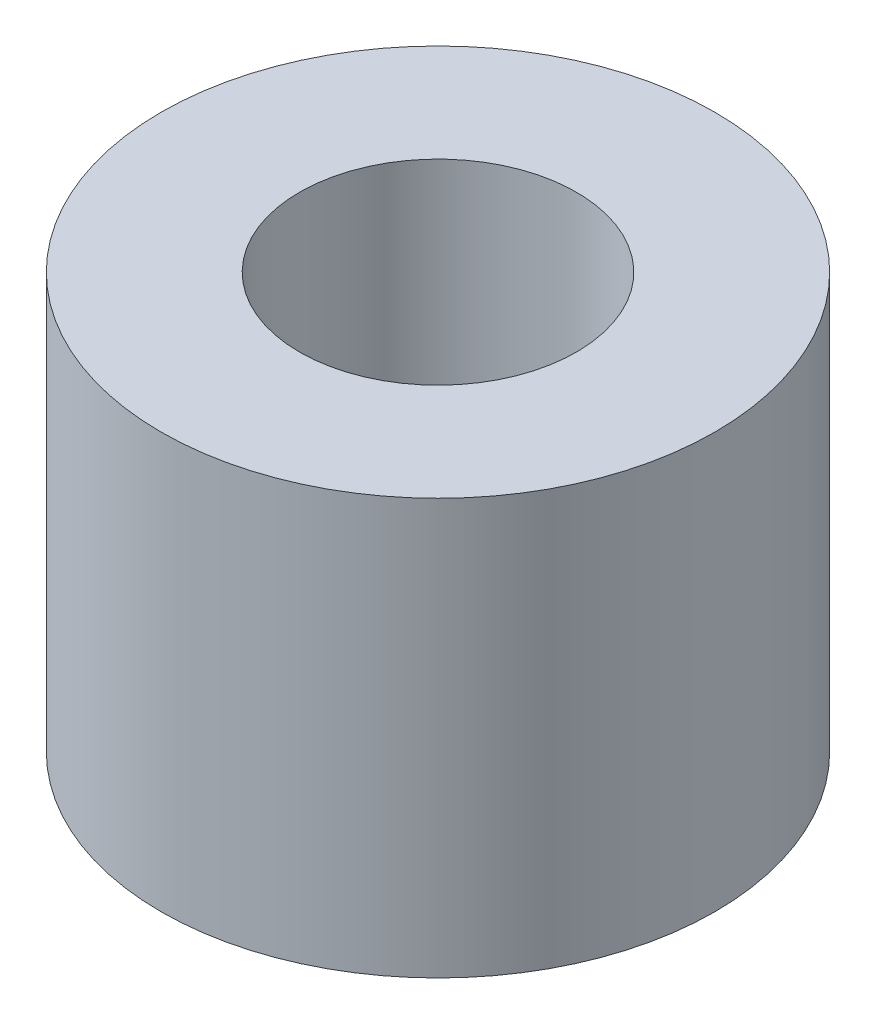
SolidWorks part; units mm, degrees
material "ABS"
ref_plane "Front Plane" through (0, 0, 0) normal (0, 0, 1) x (1, 0, 0)
ref_plane "Top Plane" through (0, 0, 0) normal (0, 1, 0) x (1, 0, 0)
ref_plane "Right Plane" through (0, 0, 0) normal (1, 0, 0) x (0, 0, -1)
sketch "Sketch1" plane through (0, 0, 0) normal (0, 0, 1) x (1, 0, 0)
  line L0 (0, 8.4164) -> (0, 0) construction
  line L2 (-2, 0) -> (-4, 0)
  line L3 (-2, 0) -> (-2, 6)
  line L4 (-2, 6) -> (-4, 6)
  line L5 (-4, 0) -> (-4, 6)
  dimension "D1" = 4
  dimension "D2" = 8
  dimension "D3" = 6
revolve "Revolve1" add sketch "Sketch1" angle 360 about L0
